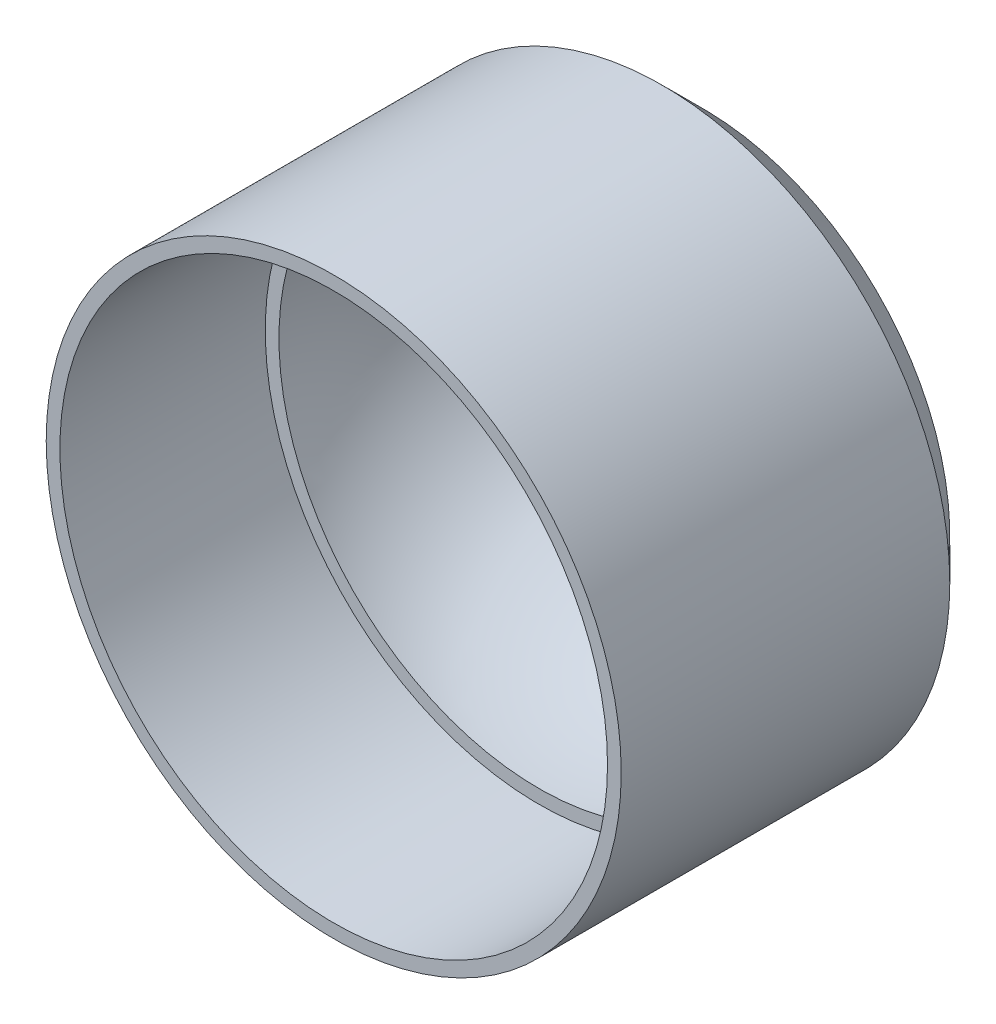
SolidWorks part; units mm, degrees
material "电镀钢"
ref_plane "Front Plane" through (0, 0, 0) normal (0, 0, 1) x (1, 0, 0)
ref_plane "Top Plane" through (0, 0, 0) normal (0, 1, 0) x (1, 0, 0)
ref_plane "Right Plane" through (0, 0, 0) normal (1, 0, 0) x (0, 0, -1)
other "Configuration Table"
sketch "Sketch1" plane through (0, 0, 0) normal (0, 0, 1) x (1, 0, 0)
  circle A1 centre (0, 0) radius 21
  dimension "D2" = 42
extrude "Boss-Extrude1" add sketch "Sketch1" along normal blind 45
sketch "Sketch2" plane through (0, 0, 45) normal (0, 0, 1) x (1, 0, 0)
  circle A0 centre (0, 0) radius 20
  dimension "D1" = 40
sketch "Sketch6" plane through (0, 0, 0) normal (0, 0, -1) x (-1, 0, 0)
  circle A0 centre (0, 0) radius 5.5
  dimension "D1" = 11
sketch "Sketch8" plane through (0, 0, 45) normal (0, 0, 1) x (1, 0, 0)
  circle A0 centre (0, 0) radius 19
  dimension "D1" = 38
extrude "Cut-Extrude4" cut sketch "Sketch8" against normal blind 15
sketch "Sketch9" plane through (0, 0, 30) normal (0, 0, 1) x (1, 0, 0)
  line L0 (19, 0) -> (-19, 0)
  circle A0 centre (0, 0) radius 19 construction
  arc A1 (19, 0) -> (-19, 0) centre (0, 0) ccw
revolve "Cut-Revolve2" cut sketch "Sketch9" angle 360 about L0
extrude "Cut-Extrude5" cut sketch "Sketch2" against normal blind 15
extrude "Cut-Extrude6" cut sketch "Sketch6" against normal through all
sketch "Sketch10" plane through (0, 0, 0) normal (0, 0, -1) x (-1, 0, 0)
  circle A0 centre (0, 0) radius 21 construction
  circle A1 centre (0, 0) radius 21
extrude "Cut-Extrude7" cut sketch "Sketch10" against normal blind 10
sketch "Sketch13" plane through (0, 0, 10) normal (0, 0, -1) x (-1, 0, 0)
  circle A0 centre (0, 0) radius 21 construction
  circle A1 centre (0, 0) radius 21
extrude "Cut-Extrude10" cut sketch "Sketch13" against normal blind 8
chamfer "Chamfer4" distance 3 1 edges at (-21, 0, 18)
